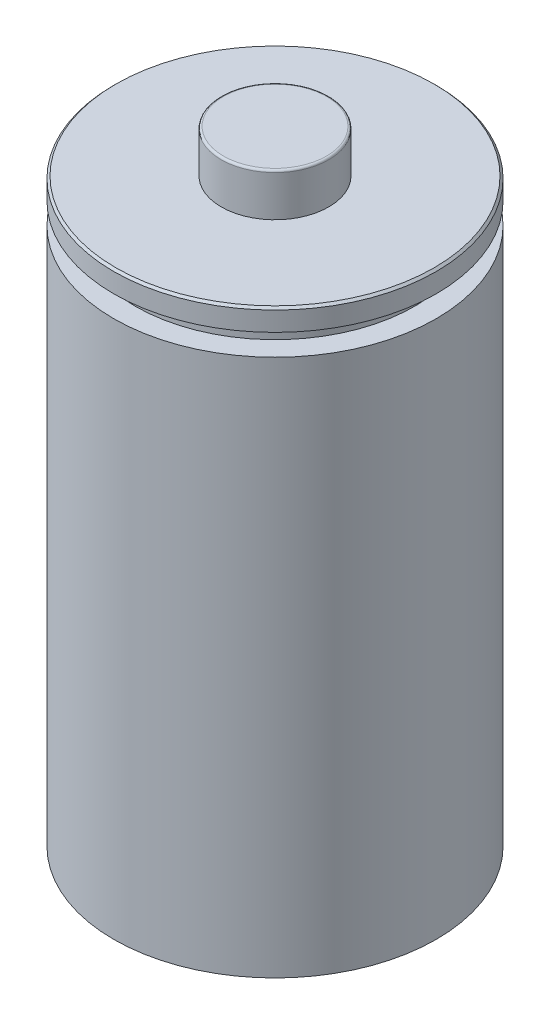
from build123d import *

# Parameters (mm, degrees)
SKETCH1_R           = 75
BOSS_EXTRUDE1_DEPTH = 250
SKETCH2_R           = 65
BOSS_EXTRUDE2_DEPTH = 10
SKETCH3_R           = 75
BOSS_EXTRUDE3_DEPTH = 10
SKETCH4_R           = 25
BOSS_EXTRUDE4_DEPTH = 20
FILLET1_R           = 1
CHAMFER1_SIZE       = 1


with BuildPart() as part:
    # Sketch1 → Boss-Extrude1 (new body)
    with BuildSketch(Plane(origin=(0, 0, 0), x_dir=(1, 0, 0), z_dir=(0, 1, 0))):
        with Locations(Location((0, 0, 0), (0, 0, 270))):
            Circle(SKETCH1_R)
    extrude(amount=BOSS_EXTRUDE1_DEPTH)

    # Sketch2 → Boss-Extrude2 (add)
    with BuildSketch(Plane(origin=(0, 250, 0), x_dir=(1, 0, 0), z_dir=(0, 1, 0))):
        with Locations(Location((0, 0, 0), (0, 0, 270))):
            Circle(SKETCH2_R)
    extrude(amount=BOSS_EXTRUDE2_DEPTH)

    # Sketch3 → Boss-Extrude3 (add)
    with BuildSketch(Plane(origin=(0, 260, 0), x_dir=(1, 0, 0), z_dir=(0, 1, 0))):
        with Locations(Location((0, 0, 0), (0, 0, 270))):
            Circle(SKETCH3_R)
    extrude(amount=BOSS_EXTRUDE3_DEPTH)

    # Sketch4 → Boss-Extrude4 (add)
    with BuildSketch(Plane(origin=(0, 270, 0), x_dir=(1, 0, 0), z_dir=(0, 1, 0))):
        with Locations(Location((0, 0, 0), (0, 0, 270))):
            Circle(SKETCH4_R)
    extrude(amount=BOSS_EXTRUDE4_DEPTH)

    # Fillet1
    fillet1_edges = [part.edges().sort_by_distance(p)[0] for p in [
        (0, 290, -25),
    ]]
    fillet(fillet1_edges, radius=FILLET1_R)

    # Chamfer1
    chamfer1_edges = [part.edges().sort_by_distance(p)[0] for p in [
        (0, 270, -75),
    ]]
    chamfer(chamfer1_edges, length=CHAMFER1_SIZE)


solid = part.part
